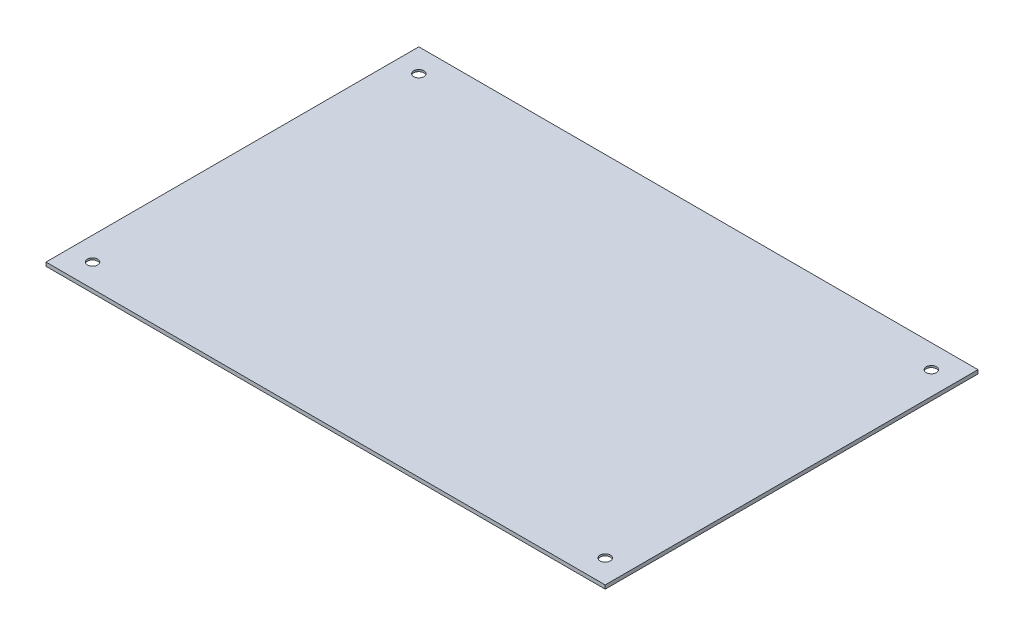
from build123d import *

# Parameters (mm, degrees)
SKETCH1_W           = 600
SKETCH1_H           = 400
BOSS_EXTRUDE1_DEPTH = 4
SHELL1_T            = -2
SKETCH2_R           = 5.5
CUT_EXTRUDE1_DEPTH  = 4


with BuildPart() as part:
    # Sketch1 → Boss-Extrude1 (new body)
    with BuildSketch(Plane(origin=(0, 0, 0), x_dir=(1, 0, 0), z_dir=(0, 1, 0))):
        Rectangle(SKETCH1_W, SKETCH1_H)
    extrude(amount=BOSS_EXTRUDE1_DEPTH)

    # Shell1
    shell1_openings = [part.faces().sort_by_distance(p)[0] for p in [
        (0, 0, 0),
    ]]
    offset(amount=SHELL1_T, openings=shell1_openings, kind=Kind.INTERSECTION)

    # Sketch2 → Cut-Extrude1 (cut)
    with BuildSketch(Plane(origin=(0, 4, 0), x_dir=(1, 0, 0), z_dir=(0, 1, 0))):
        with Locations(Location((-275, 175, 0), (0, 0, 270))):
            Circle(SKETCH2_R)
        with Locations(Location((275, 175, 0), (0, 0, 270))):
            Circle(SKETCH2_R)
        with Locations(Location((275, -175, 0), (0, 0, 270))):
            Circle(SKETCH2_R)
        with Locations(Location((-275, -175, 0), (0, 0, 270))):
            Circle(SKETCH2_R)
    extrude(amount=-CUT_EXTRUDE1_DEPTH, mode=Mode.SUBTRACT)


solid = part.part
